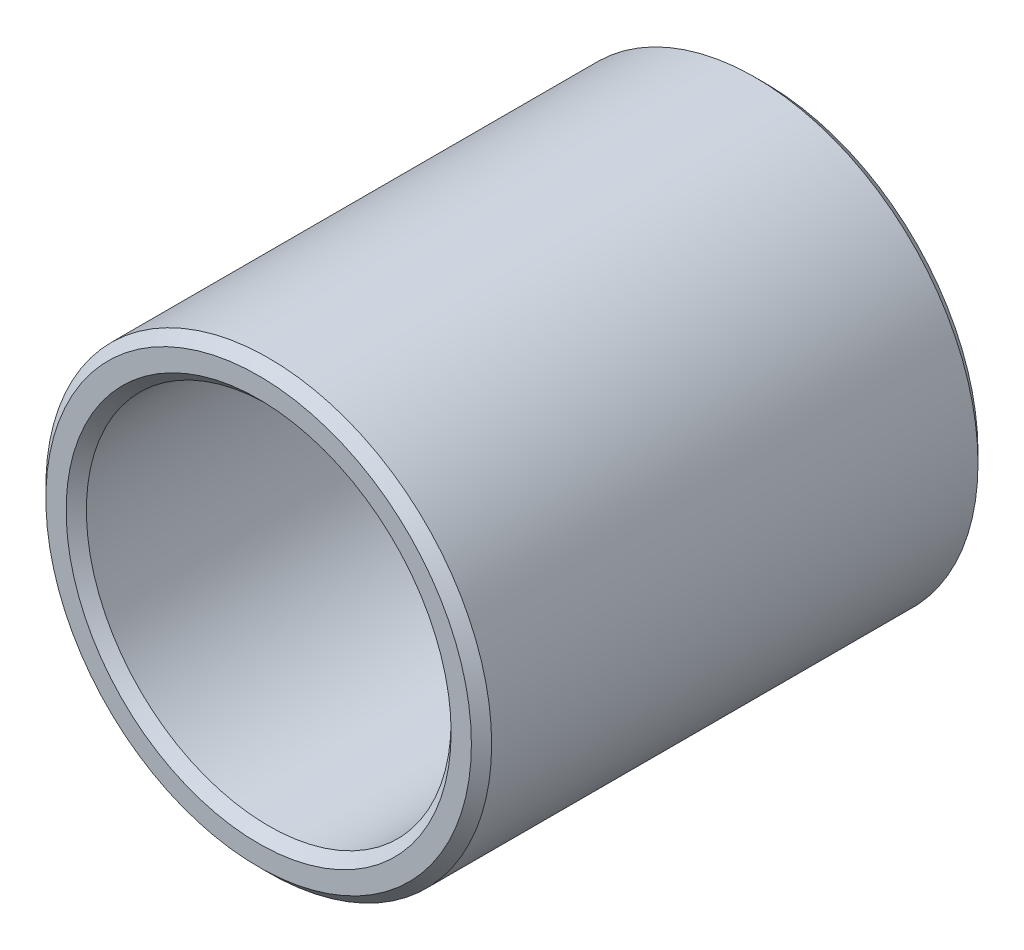
from build123d import *

# Parameters (mm, degrees)
SKETCH_1_R      = 11
SKETCH_1_R_2    = 9
EXTRUDE_1_DEPTH = 25
CHAMFER_1_SIZE  = 0.5


with BuildPart() as part:
    # 草图1 → 凸台-拉伸1 (new body)
    with BuildSketch(Plane.XY):
        Circle(SKETCH_1_R)
        Circle(SKETCH_1_R_2, mode=Mode.SUBTRACT)
    extrude(amount=EXTRUDE_1_DEPTH)

    # 倒角1
    chamfer_1_edges = [part.edges().sort_by_distance(p)[0] for p in [
        (-11, 0, 0),
        (-11, 0, 25),
        (-9, 0, 0),
        (-9, 0, 25),
    ]]
    chamfer(chamfer_1_edges, length=CHAMFER_1_SIZE)


solid = part.part
